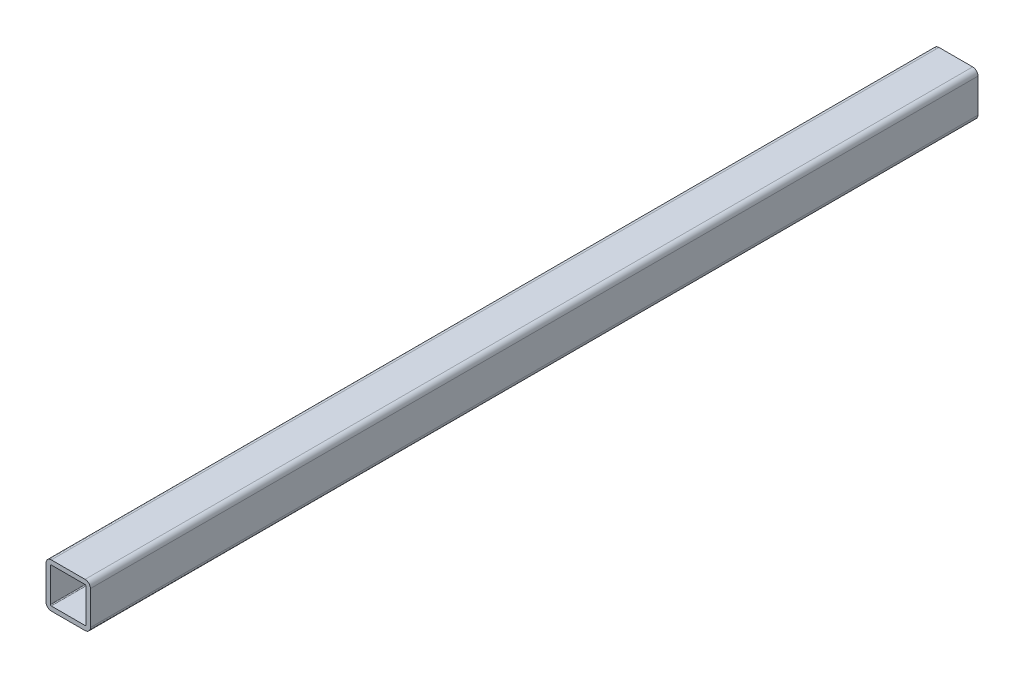
from build123d import *

# Parameters (mm, degrees)
BOSS_EXTRUDE1_DEPTH = 1000


with BuildPart() as part:
    # Sketch1 → Boss-Extrude1 (new body)
    with BuildSketch(Plane.XY):
        with BuildLine():
            Line((6, 0), (44, 0))
            ThreePointArc((44, 0), (48.242640687, 1.757359313), (50, 6))
            Line((50, 6), (50, 44))
            ThreePointArc((50, 44), (48.242640687, 48.242640687), (44, 50))
            Line((44, 50), (6, 50))
            ThreePointArc((6, 50), (1.757359313, 48.242640687), (0, 44))
            Line((0, 44), (0, 6))
            ThreePointArc((0, 6), (1.757359313, 1.757359313), (6, 0))
        make_face()
        with BuildLine():
            Line((6, 45), (44, 45))
            ThreePointArc((44, 45), (44.707106781, 44.707106781), (45, 44))
            Line((45, 44), (45, 6))
            ThreePointArc((45, 6), (44.707106781, 5.292893219), (44, 5))
            Line((44, 5), (6, 5))
            ThreePointArc((6, 5), (5.292893219, 5.292893219), (5, 6))
            Line((5, 6), (5, 44))
            ThreePointArc((5, 44), (5.292893219, 44.707106781), (6, 45))
        make_face(mode=Mode.SUBTRACT)
    extrude(amount=BOSS_EXTRUDE1_DEPTH)


solid = part.part
